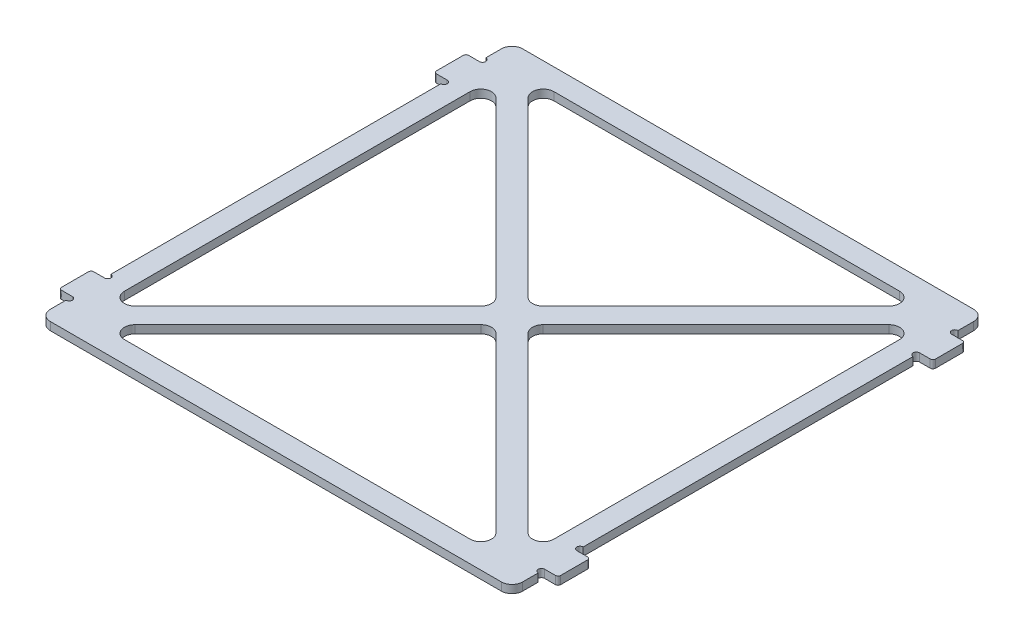
SolidWorks part; units mm, degrees
material "Thornel Mat VMA"
ref_plane "前视基准面" through (0, 0, 0) normal (0, 0, 1) x (1, 0, 0)
ref_plane "上视基准面" through (0, 0, 0) normal (0, 1, 0) x (1, 0, 0)
ref_plane "右视基准面" through (0, 0, 0) normal (1, 0, 0) x (0, 0, -1)
other "Configuration Table"
sketch "草图1" plane through (0, 0, 0) normal (0, 1, 0) x (1, 0, 0)
  line L0 (0, 0) -> (51.6848, 0) construction
  line L1 (-44.1, 44.1) -> (44.1, 44.1)
  line L2 (-44.1, 44.1) -> (-44.1, -44.1)
  line L3 (-44.1, -44.1) -> (44.1, -44.1)
  line L4 (44.1, 44.1) -> (44.1, -44.1)
  line L5 (-44.1, 44.1) -> (44.1, -44.1) construction
  line L6 (-44.1, -44.1) -> (44.1, 44.1) construction
  line L7 (0, 0) -> (0, 52.4021) construction
  line L8 (44.1, -32) -> (46.6, -32)
  line L9 (44.1, 38) -> (46.6, 38)
  line L10 (44.1, 38) -> (44.1, 32)
  line L11 (44.1, 32) -> (46.6, 32)
  line L12 (46.6, 38) -> (46.6, 32)
  line L13 (46.6, -38) -> (46.6, -32)
  line L14 (44.1, -38) -> (46.6, -38)
  line L15 (-44.1, -38) -> (-46.6, -38)
  line L16 (-46.6, -38) -> (-46.6, -32)
  line L17 (-44.1, -32) -> (-46.6, -32)
  line L18 (-44.1, 32) -> (-46.6, 32)
  line L19 (-44.1, 38) -> (-46.6, 38)
  line L20 (-46.6, 38) -> (-46.6, 32)
  line L21 (-37.1, 40.1) -> (0, 3)
  line L22 (-40.1, 40.1) -> (40.1, 40.1)
  line L23 (-40.1, 40.1) -> (-40.1, -40.1)
  line L24 (-40.1, -40.1) -> (40.1, -40.1)
  line L25 (40.1, 40.1) -> (40.1, -40.1)
  line L26 (-40.1, 40.1) -> (40.1, -40.1) construction
  line L27 (-40.1, -40.1) -> (40.1, 40.1) construction
  line L28 (0, 3) -> (37.1, 40.1)
  line L29 (3, 0) -> (40.1, 37.1)
  line L30 (40.1, -37.1) -> (3, 0)
  line L31 (37.1, -40.1) -> (0, -3)
  line L32 (0, -3) -> (-37.1, -40.1)
  line L33 (-40.1, 37.1) -> (-3, 0)
  line L34 (-3, 0) -> (-40.1, -37.1)
  circle A0 centre (44.1, 38.6) radius 0.6
  circle A1 centre (44.1, 31.4) radius 0.6
  circle A2 centre (44.1, -31.4) radius 0.6
  circle A3 centre (44.1, -38.6) radius 0.6
  circle A4 centre (-44.1, -31.4) radius 0.6
  circle A5 centre (-44.1, -38.6) radius 0.6
  circle A6 centre (-44.1, 31.4) radius 0.6
  circle A7 centre (-44.1, 38.6) radius 0.6
  point P0 (0, 0)
  point P47 (-30.2563, 36)
  point P58 (31.383, 36)
  dimension "D6" = 1.2
  dimension "D1" = 6
  dimension "D2" = 2.5
  dimension "D3" = 6.1
  dimension "D4" = 70
  dimension "D5" = 88.2
  dimension "D7" = 4
  dimension "D8" = 4
  dimension "D9" = 3
extrude "凸台-拉伸1" add sketch "草图1" along normal blind 1.5
fillet "圆角1" radius 0.5 8 edges at (46.6, 0.75, -32) (46.6, 0.75, -38) (46.6, 0.75, 32) (46.6, 0.75, 38) (-46.6, 0.75, 38) (-46.6, 0.75, 32) (-46.6, 0.75, -32) (-46.6, 0.75, -38)
fillet "圆角2" radius 2 16 edges at (37.1, 0.75, 40.1) (-37.1, 0.75, 40.1) (0, 0.75, 3) (37.1, 0.75, -40.1) (-37.1, 0.75, -40.1) (0, 0.75, -3) (40.1, 0.75, 37.1) (40.1, 0.75, -37.1) (3, 0.75, 0) (-3, 0.75, 0) (-40.1, 0.75, -37.1) (-40.1, 0.75, 37.1) (-44.1, 0.75, 44.1) (-44.1, 0.75, -44.1) (44.1, 0.75, -44.1) (44.1, 0.75, 44.1)
